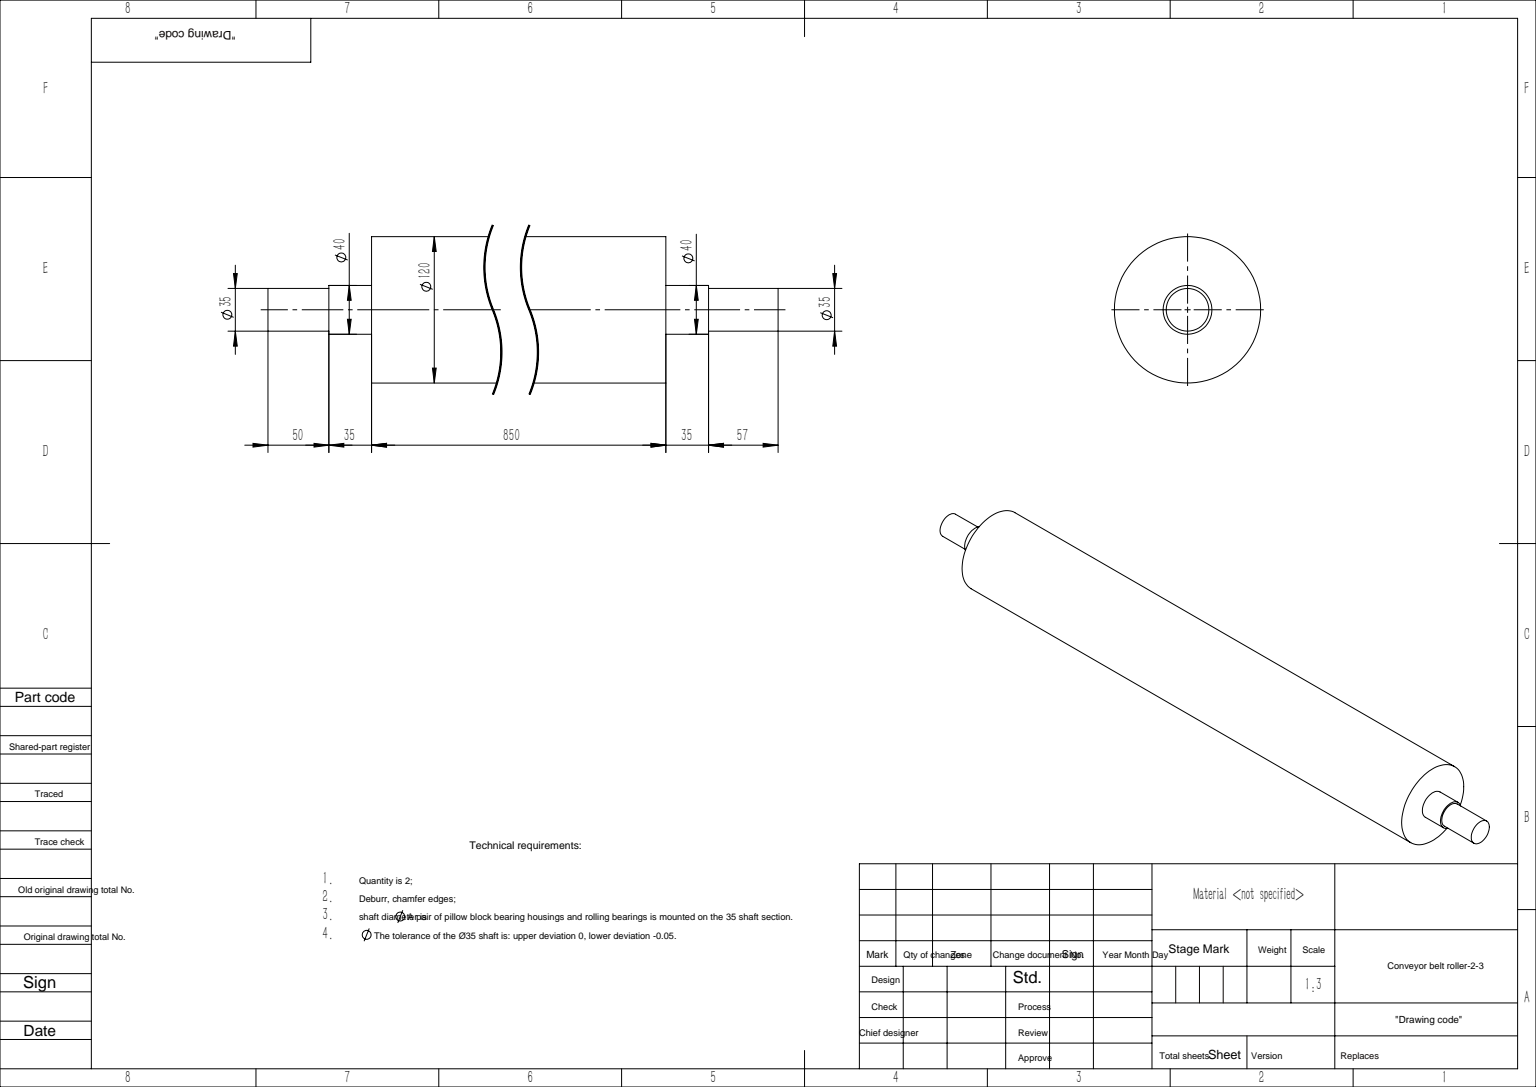
from build123d import *


with BuildPart() as part:
    # 草图1 → 旋转1 (revolve)
    with BuildSketch(Plane.XY, mode=Mode.PRIVATE) as revolve_1_sk:
        Polygon((0, 0), (0, 17.5), (50, 17.5), (50, 20), (85, 20), (85, 60), (935, 60), (935, 20), (970, 20), (970, 17.5), (1027, 17.5), (1027, 0), align=None)
    revolve(revolve_1_sk.sketch.rotate(Axis((1027, 0, 0), (-1, 0, 0)), 90), axis=Axis((1027, 0, 0), (-1, 0, 0)))


solid = part.part
